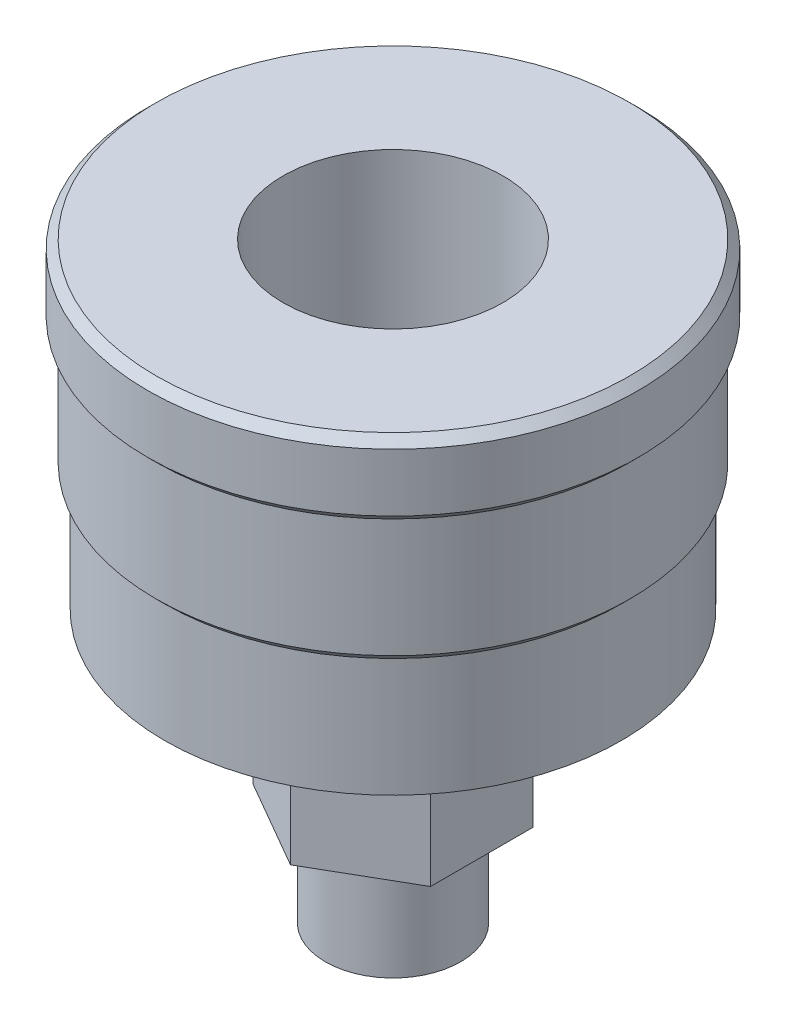
SolidWorks part; units mm, degrees
material "Q235"
ref_plane "Front Plane" through (0, 0, 0) normal (0, 0, 1) x (1, 0, 0)
ref_plane "Top Plane" through (0, 0, 0) normal (0, 1, 0) x (1, 0, 0)
ref_plane "Right Plane" through (0, 0, 0) normal (1, 0, 0) x (0, 0, -1)
sketch "Sketch1" plane through (0, 0, 0) normal (0, 0, 1) x (1, 0, 0)
  line L0 (-28, 70) -> (-29, 69)
  line L1 (-29, 62.153) -> (-29, 69)
  line L2 (-2.5, 0) -> (-2.5, 32.153)
  line L3 (-29, 62.153) -> (-28, 61.153)
  line L4 (-28, 61.153) -> (-28, 47.153)
  line L5 (-28, 47.153) -> (-27, 46.153)
  line L6 (-27, 46.153) -> (-27, 32.153)
  line L7 (-27, 32.153) -> (-25, 32.153)
  line L8 (-25, 32.153) -> (-10.5, 22)
  line L9 (-10.5, 22) -> (-10.5, 12)
  line L10 (-10.5, 12) -> (-8, 10.6986)
  line L11 (-8, 10.6986) -> (-8, 0)
  line L12 (-8, 0) -> (-2.5, 0)
  line L13 (0, 0) -> (0, -5.3853) construction
  line L14 (-2.5, 32.153) -> (-13.0031, 47.153)
  line L15 (-13.0031, 47.153) -> (-13.0031, 70)
  line L16 (-13.0031, 70) -> (-28, 70)
  dimension "d" = 16
  dimension "D2" = 1
  dimension "d1" = 5
  dimension "D3" = 117.5
  dimension "D4" = 1
  dimension "l" = 12
  dimension "D5" = 45
  dimension "h1" = 10
  dimension "D6" = 45
  dimension "dm" = 54
  dimension "hm" = 30
  dimension "lm" = 70
  dimension "D9" = 55
  dimension "sm" = 21
  dimension "D10" = 35
  dimension "D11" = 45
  dimension "D12" = 1
  dimension "D13" = 2
revolve "Revolve1" add sketch "Sketch1" angle 360 about L13
ref_plane "Plane1" through (0, 12, 0) normal (0, 1, 0) x (-1, 0, 0)
sketch "Sketch2" plane through (0, 12, 0) normal (0, 1, 0) x (-1, 0, 0)
  line L1 (-10.5, 6.0622) -> (-10.5, -6.0622)
  line L2 (-10.5, -6.0622) -> (0, -12.1244)
  line L3 (0, -12.1244) -> (10.5, -6.0622)
  line L4 (10.5, -6.0622) -> (10.5, 6.0622)
  line L5 (10.5, 6.0622) -> (0, 12.1244)
  line L6 (0, 12.1244) -> (-10.5, 6.0622)
  circle A0 centre (0, 0) radius 10.5 construction
  circle A1 centre (0, 0) radius 10.5 construction
extrude "Extrude1" add sketch "Sketch2" along normal up to vertex (20.153 mm away) up to point (-25, 32.153, 0)
